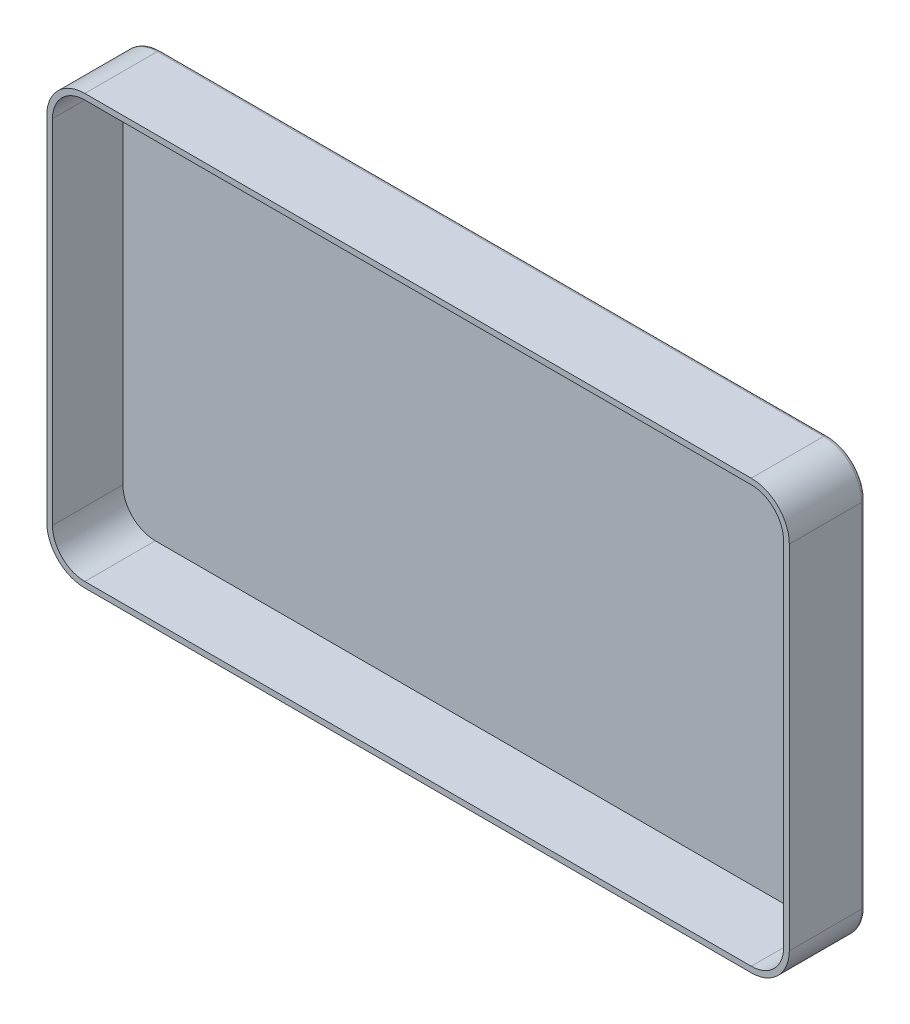
SolidWorks part; units mm, degrees
ref_plane "前视" through (0, 0, 0) normal (0, 0, 1) x (1, 0, 0)
ref_plane "上视" through (0, 0, 0) normal (0, 1, 0) x (1, 0, 0)
ref_plane "右视" through (0, 0, 0) normal (1, 0, 0) x (0, 0, -1)
sketch "草图1" plane through (0, 0, 0) normal (0, 0, 1) x (1, 0, 0)
  line L1 (-195, -112.5) -> (195, -112.5)
  line L2 (-195, -112.5) -> (-195, 112.5)
  line L3 (-195, 112.5) -> (195, 112.5)
  line L4 (195, -112.5) -> (195, 112.5)
  line L5 (-195, -112.5) -> (195, 112.5) construction
  line L6 (-195, 112.5) -> (195, -112.5) construction
  point P0 (0, 0)
  dimension "D1" = 390
  dimension "D2" = 225
extrude "凸台-拉伸1" add sketch "草图1" along normal blind 40
fillet "圆角1" radius 20 4 edges at (195, -112.5, 20) (-195, 112.5, 20) (195, 112.5, 20) (-195, -112.5, 20)
shell "抽壳1" thickness 3
fillet "圆角2" radius 2 8 edges at (189.1421, 106.6421, 0) (0, 112.5, 0) (-189.1421, 106.6421, 0) (-195, 0, 0) (-189.1421, -106.6421, 0) (0, -112.5, 0) (189.1421, -106.6421, 0) (195, 0, 0)
sketch "草图2" plane through (0, 0, 0) normal (0, 0, -1) x (-1, 0, 0)
  line L1 (-130, -65) -> (130, -65) construction
  line L2 (-130, -65) -> (-130, 65) construction
  line L3 (-130, 65) -> (130, 65) construction
  line L4 (130, -65) -> (130, 65) construction
  line L5 (-130, -65) -> (130, 65) construction
  line L6 (-130, 65) -> (130, -65) construction
  circle A1 centre (-130, 65) radius 7.5
  point P0 (0, 0)
  dimension "D3" = 15
  dimension "D1" = 260
  dimension "D2" = 130
extrude "凸台-拉伸2" add sketch "草图2" along normal blind 8
fillet "圆角3" radius 2 1 edges at (122.5, 65, -8)
pattern_linear "阵列(线性)1" count 2 spacing 260 along (-1, 0, 0) count 2 spacing 130 along (0, -1, 0) of "凸台-拉伸2", "圆角3"
